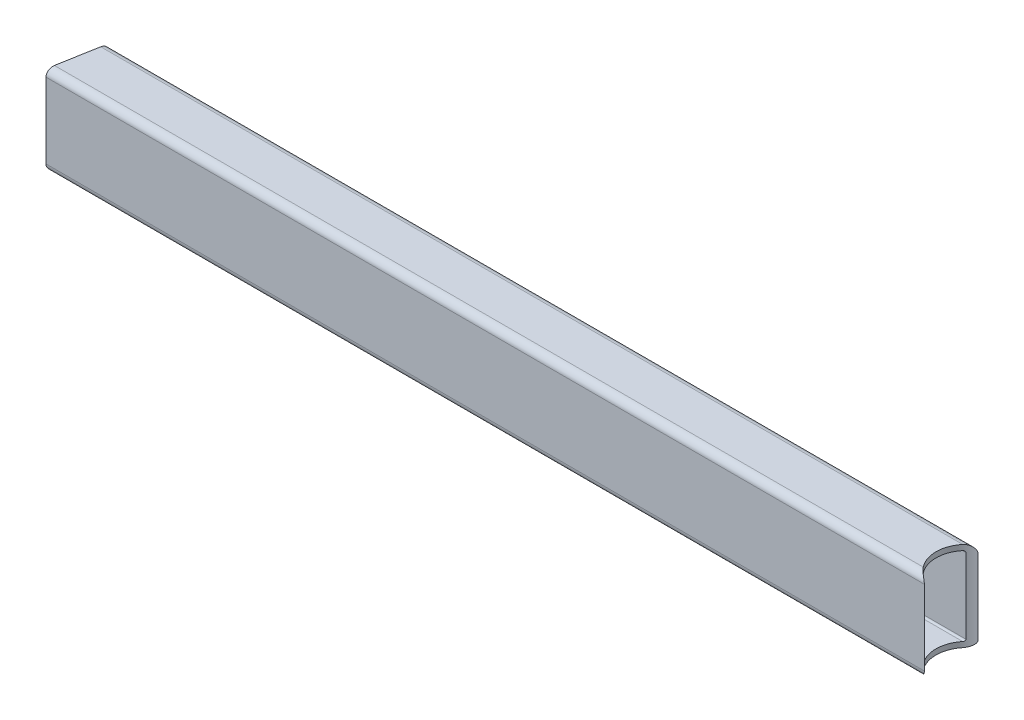
from build123d import *

# Parameters (mm, degrees)
SQUARE_TUBE_30_X_30_X_2_6_15_DEPTH = 600
CUT_EXTRUDE3_DEPTH                 = 113
SKETCH13_R                         = 17.5
CUT_EXTRUDE4_DEPTH                 = 113


with BuildPart() as part:
    # Sketch1 → Square tube 30 X 30 X 2.6(15) (new body)
    with BuildSketch(Plane(origin=(0, 0, 0), x_dir=(0, -1, 0), z_dir=(-1, 0, 0))):
        with BuildLine():
            Line((-21, -15), (21, -15))
            ThreePointArc((21, -15), (23.828427125, -13.828427125), (25, -11))
            Line((25, -11), (25, 11))
            ThreePointArc((25, 11), (23.828427125, 13.828427125), (21, 15))
            Line((21, 15), (-21, 15))
            ThreePointArc((-21, 15), (-23.828427125, 13.828427125), (-25, 11))
            Line((-25, 11), (-25, -11))
            ThreePointArc((-25, -11), (-23.828427125, -13.828427125), (-21, -15))
        make_face()
        with BuildLine():
            Line((-21, -12), (21, -12))
            ThreePointArc((21, -12), (21.707106781, -11.707106781), (22, -11))
            Line((22, -11), (22, 11))
            ThreePointArc((22, 11), (21.707106781, 11.707106781), (21, 12))
            Line((21, 12), (-21, 12))
            ThreePointArc((-21, 12), (-21.707106781, 11.707106781), (-22, 11))
            Line((-22, 11), (-22, -11))
            ThreePointArc((-22, -11), (-21.707106781, -11.707106781), (-21, -12))
        make_face(mode=Mode.SUBTRACT)
    extrude(amount=SQUARE_TUBE_30_X_30_X_2_6_15_DEPTH)

    # Sketch12 → Cut-Extrude3 (cut)
    with BuildSketch(Plane.XZ.offset(25)):
        Polygon((-500, 15), (-494.710190579, -15), (-600, -15), (-600, 15), align=None)
    extrude(amount=-CUT_EXTRUDE3_DEPTH, mode=Mode.SUBTRACT)

    # Sketch13 → Cut-Extrude4 (cut)
    with BuildSketch(Plane.XZ.offset(25)):
        Circle(SKETCH13_R)
    extrude(amount=-CUT_EXTRUDE4_DEPTH, mode=Mode.SUBTRACT)


solid = part.part
